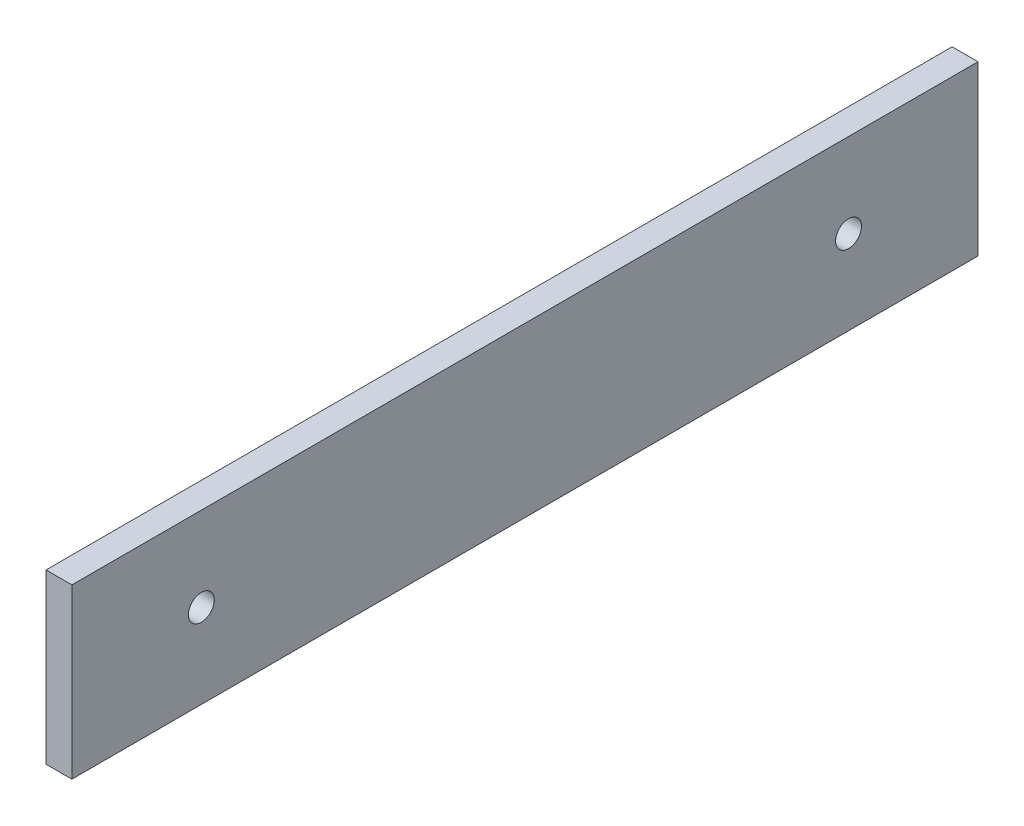
SolidWorks part; units mm, degrees
ref_plane "Front Plane" through (0, 0, 0) normal (0, 0, 1) x (1, 0, 0)
ref_plane "Top Plane" through (0, 0, 0) normal (0, 1, 0) x (1, 0, 0)
ref_plane "Right Plane" through (0, 0, 0) normal (1, 0, 0) x (0, 0, -1)
other "Configuration Table"
sketch "Sketch1" plane through (0, 0, 0) normal (1, 0, 0) x (0, 0, -1)
  line L0 (-350, 0) -> (350, 0) construction
  line L1 (-350, 65) -> (350, 65)
  line L2 (-350, 65) -> (-350, -65)
  line L3 (-350, -65) -> (350, -65)
  line L4 (350, 65) -> (350, -65)
  line L5 (-350, 65) -> (350, -65) construction
  line L6 (-350, -65) -> (350, 65) construction
  circle A0 centre (-250, 0) radius 10
  circle A1 centre (250, 0) radius 10
  point P0 (0, 0)
  dimension "D1" = 500
  dimension "D2" = 250
  dimension "D4" = 20
  dimension "D5" = 20
  dimension "D3" = 130
  dimension "D6" = 700
extrude "Boss-Extrude1" add sketch "Sketch1" along normal blind 20
